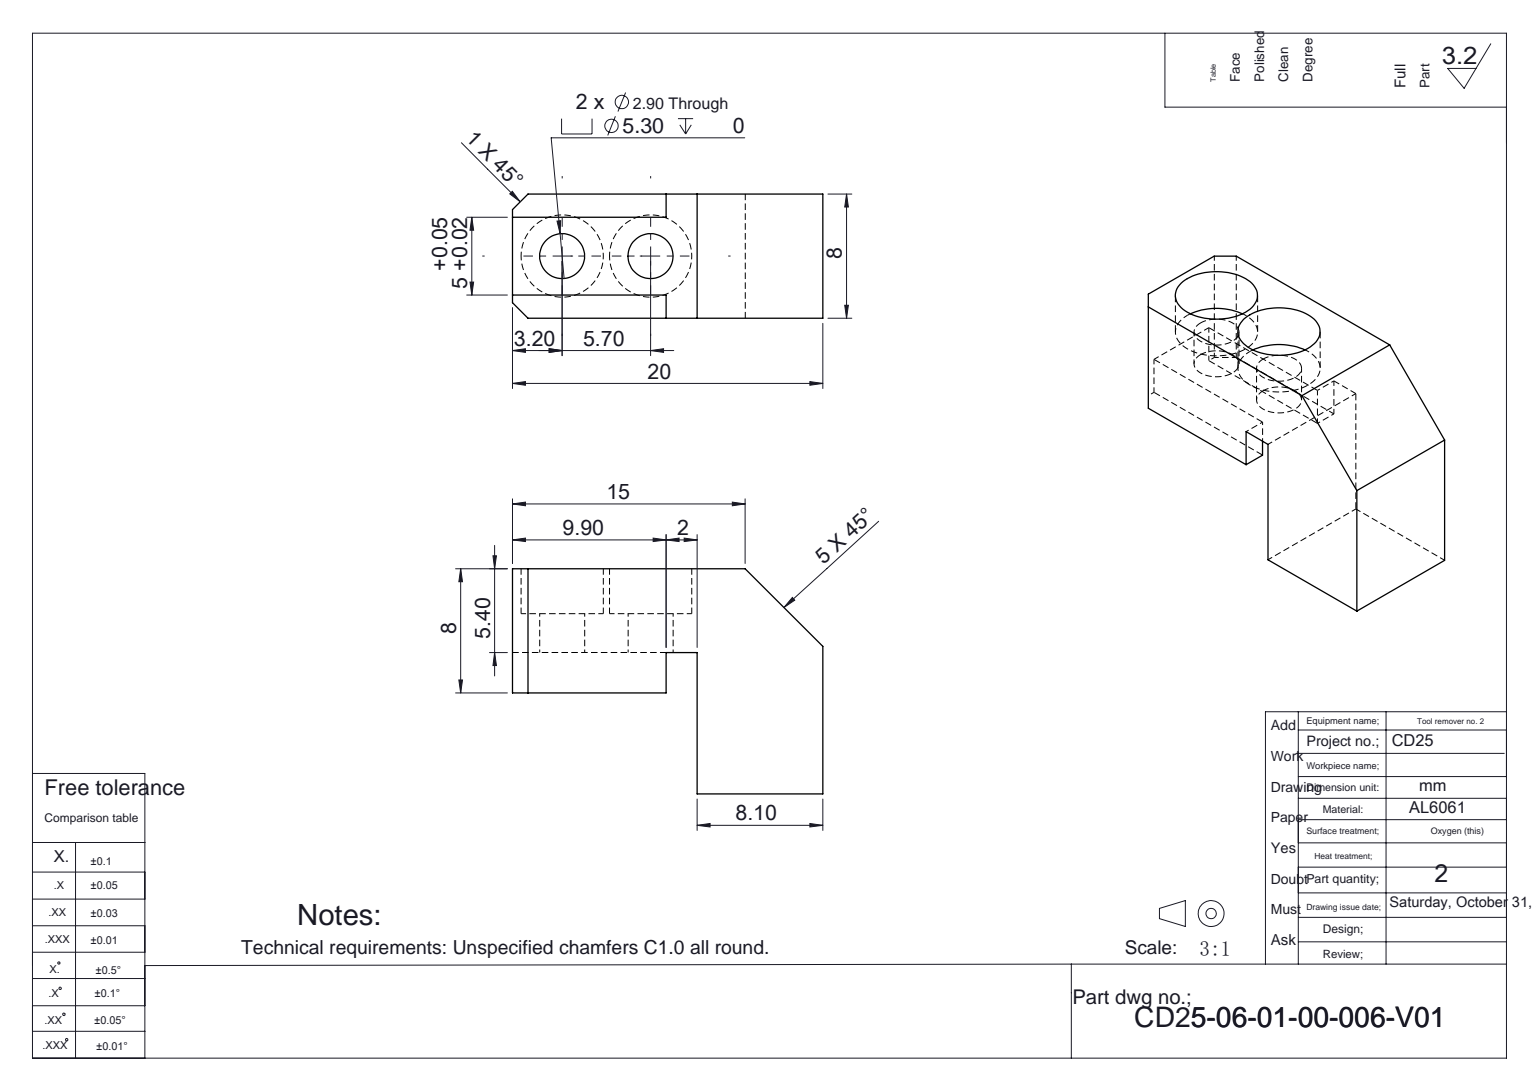
from build123d import *

# Parameters (mm, degrees)
SKETCH1_W                                            = 8
SKETCH1_H                                            = 20
BOSS_EXTRUDE1_DEPTH                                  = 7.25
SKETCH2_W                                            = 5
SKETCH2_H                                            = 11.9
CUT_EXTRUDE1_DEPTH                                   = 9.1
CBORE_FOR_M2_5_HEX_SOCKET_HEAD_CAP_SCREW_D           = 2.9
CBORE_FOR_M2_5_HEX_SOCKET_HEAD_CAP_SCREW_CBORE_D     = 5.3
CBORE_FOR_M2_5_HEX_SOCKET_HEAD_CAP_SCREW_CBORE_DEPTH = 2.9
SKETCH7_W                                            = 11.4
SKETCH7_H                                            = 6.5
CUT_EXTRUDE3_DEPTH                                   = 15.716062653
CHAMFER1_SIZE                                        = 1
CHAMFER2_SIZE                                        = 5
CUT_EXTRUDE4_DEPTH                                   = 9.1


with BuildPart() as part:
    # Sketch1 → Boss-Extrude1 (new, symmetric)
    with BuildSketch(Plane(origin=(0, 0, 0), x_dir=(1, 0, 0), z_dir=(0, 1, 0))):
        Rectangle(SKETCH1_W, SKETCH1_H)
    extrude(amount=BOSS_EXTRUDE1_DEPTH, both=True)

    # Sketch2 → Cut-Extrude1 (cut)
    with BuildSketch(Plane.XZ.offset(7.25)):
        with Locations((0, 4.05)):
            Rectangle(SKETCH2_W, SKETCH2_H)
    extrude(amount=-CUT_EXTRUDE1_DEPTH, mode=Mode.SUBTRACT)

    # CBORE for M2.5 Hex Socket Head Cap Screw2 (through all)
    with Locations(Plane(origin=(0, 7.25, 0), x_dir=(1, 0, 0), z_dir=(0, 1, 0))):
        with Locations((0, -6.8), (0, -1.1)):
            CounterBoreHole(CBORE_FOR_M2_5_HEX_SOCKET_HEAD_CAP_SCREW_D / 2, CBORE_FOR_M2_5_HEX_SOCKET_HEAD_CAP_SCREW_CBORE_D / 2, CBORE_FOR_M2_5_HEX_SOCKET_HEAD_CAP_SCREW_CBORE_DEPTH)

    # Sketch7 → Cut-Extrude3 (cut, through all)
    with BuildSketch(Plane(origin=(4, 0, 0), x_dir=(0, 0, -1), z_dir=(1, 0, 0))):
        with Locations((-4.3, -4)):
            Rectangle(SKETCH7_W, SKETCH7_H)
    extrude(amount=-CUT_EXTRUDE3_DEPTH, mode=Mode.SUBTRACT)

    # Chamfer1
    chamfer1_edges = [part.edges().sort_by_distance(p)[0] for p in [
        (4, 3.25, 10),
        (-4, 3.25, 10),
    ]]
    chamfer(chamfer1_edges, length=CHAMFER1_SIZE)

    # Chamfer2
    chamfer2_edges = [part.edges().sort_by_distance(p)[0] for p in [
        (0, 7.25, -10),
    ]]
    chamfer(chamfer2_edges, length=CHAMFER2_SIZE)

    # Sketch6 → Cut-Extrude4 (cut)
    with BuildSketch(Plane.XZ.offset(7.25)):
        with BuildLine():
            Line((-4, 0.1), (4, 0.1))
            ThreePointArc((4, 0.1), (5, -0.9), (4, -1.9))
            Line((4, -1.9), (-4, -1.9))
            ThreePointArc((-4, -1.9), (-5, -0.9), (-4, 0.1))
        make_face()
    extrude(amount=-CUT_EXTRUDE4_DEPTH, mode=Mode.SUBTRACT)


solid = part.part
